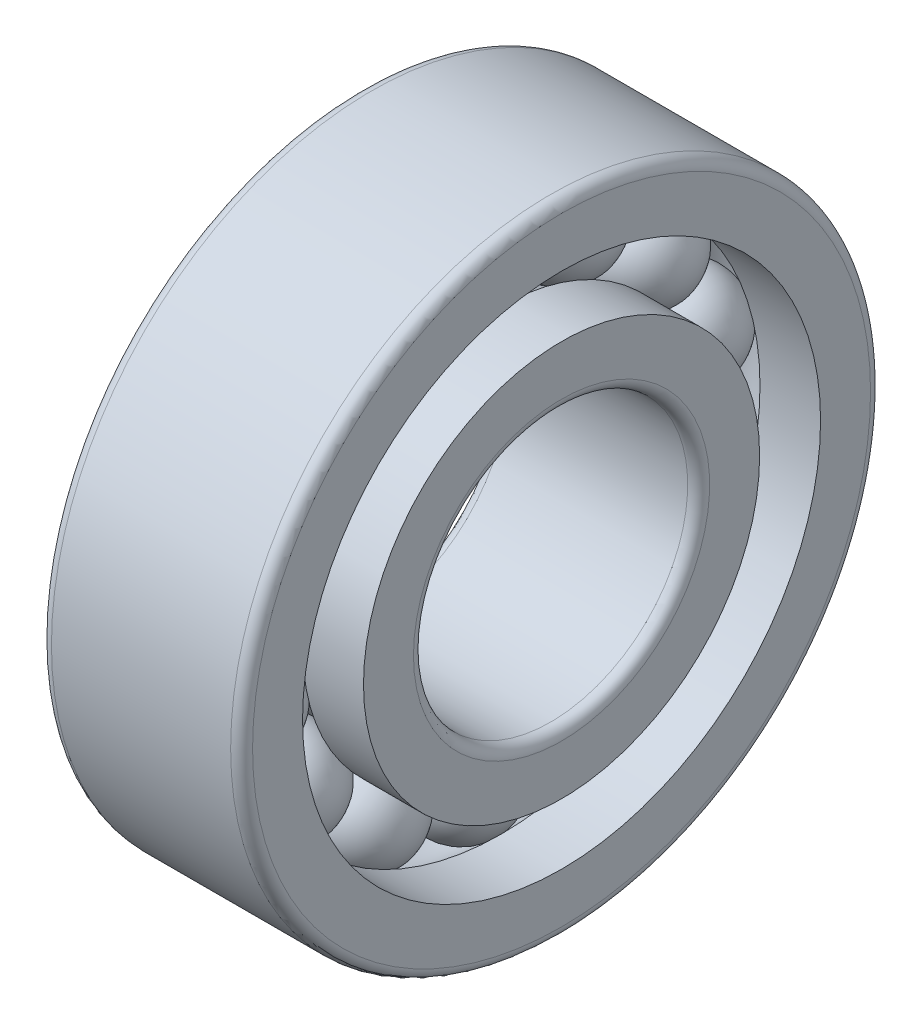
from build123d import *

# Parameters (mm, degrees)
PATTERN_CIRCULAR_5_COUNT = 14


with BuildPart() as part:
    # 草图2 → 旋转1 (revolve)
    with BuildSketch(Plane.XY, mode=Mode.PRIVATE) as revolve_1_sk:
        with BuildLine():
            Line((-5.2, 10.833333333), (-5.5, 10.833333333))
            Line((-5.5, 10.833333333), (-5.5, 10.233333333))
            Line((-5.5, 10.233333333), (-5.5, 8.1))
            ThreePointArc((-5.5, 8.1), (-5.324264069, 7.675735931), (-4.9, 7.5))
            Line((-4.9, 7.5), (4.9, 7.5))
            ThreePointArc((4.9, 7.5), (5.324264069, 7.675735931), (5.5, 8.1))
            Line((5.5, 8.1), (5.5, 10.233333333))
            Line((5.5, 10.233333333), (5.5, 10.833333333))
            Line((5.5, 10.833333333), (4.9, 10.833333333))
            Line((4.9, 10.833333333), (2.187400791, 10.833333333))
            ThreePointArc((2.187400791, 10.833333333), (0, 9.75), (-2.187400791, 10.833333333))
            Line((-2.187400791, 10.833333333), (-4, 10.833333333))
            Line((-4, 10.833333333), (-4, 10.233333333))
            Line((-4, 10.233333333), (-4.6, 10.233333333))
            Line((-4.6, 10.233333333), (-5.2, 10.833333333))
        make_face()
        with BuildLine():
            Line((-5.5, 14.166666667), (-5.2, 14.166666667))
            Line((-5.2, 14.166666667), (-4.6, 14.766666667))
            Line((-4.6, 14.766666667), (-4, 14.766666667))
            Line((-4, 14.766666667), (-4, 14.166666667))
            Line((-4, 14.166666667), (-2.187400791, 14.166666667))
            ThreePointArc((-2.187400791, 14.166666667), (0, 15.25), (2.187400791, 14.166666667))
            Line((2.187400791, 14.166666667), (5.5, 14.166666667))
            Line((5.5, 14.166666667), (5.5, 16.9))
            ThreePointArc((5.5, 16.9), (5.324264069, 17.324264069), (4.9, 17.5))
            Line((4.9, 17.5), (-4.9, 17.5))
            ThreePointArc((-4.9, 17.5), (-5.324264069, 17.324264069), (-5.5, 16.9))
            Line((-5.5, 16.9), (-5.5, 14.166666667))
        make_face()
    revolve(revolve_1_sk.sketch.rotate(Axis((-3.5, 0, 0), (1, 0, 0)), 90), axis=Axis((-3.5, 0, 0), (1, 0, 0)))


with BuildPart() as body_2:
    # 草图3 → 旋转2 (revolve)
    with BuildSketch(Plane.XY):
        with BuildLine():
            Line((-2.75, 12.5), (2.75, 12.5))
            ThreePointArc((2.75, 12.5), (0, 15.25), (-2.75, 12.5))
        make_face()
    revolve(axis=Axis((2.75, 12.5, 0), (1, 0, 0)))


with BuildPart() as body_3:
    # 草图4 → 旋转3 (revolve)
    with BuildSketch(Plane.XY, mode=Mode.PRIVATE) as revolve_3_sk:
        Polygon((-5.2, 14.166666667), (-5.2, 10.833333333), (-4.6, 10.233333333), (-4, 10.233333333), (-4, 10.833333333), (-4.6, 11.433333333), (-4.6, 13.566666667), (-4, 14.166666667), (-4, 14.766666667), (-4.6, 14.766666667), align=None)
    revolve(revolve_3_sk.sketch.rotate(Axis((-19.927092192, 0, 0), (1, 0, 0)), 90), axis=Axis((-19.927092192, 0, 0), (1, 0, 0)))


with BuildPart() as pattern_circular_5_1:
    # 阵列(圆周)5: pattern copy
    add(body_2.part.rotate(Axis((0, 0, 0), (1, 0, 0)), 1 * 360 / PATTERN_CIRCULAR_5_COUNT))


with BuildPart() as pattern_circular_5_2:
    # 阵列(圆周)5: pattern copy
    add(body_2.part.rotate(Axis((0, 0, 0), (1, 0, 0)), 2 * 360 / PATTERN_CIRCULAR_5_COUNT))


with BuildPart() as pattern_circular_5_3:
    # 阵列(圆周)5: pattern copy
    add(body_2.part.rotate(Axis((0, 0, 0), (1, 0, 0)), 3 * 360 / PATTERN_CIRCULAR_5_COUNT))


with BuildPart() as pattern_circular_5_4:
    # 阵列(圆周)5: pattern copy
    add(body_2.part.rotate(Axis((0, 0, 0), (1, 0, 0)), 4 * 360 / PATTERN_CIRCULAR_5_COUNT))


with BuildPart() as pattern_circular_5_5:
    # 阵列(圆周)5: pattern copy
    add(body_2.part.rotate(Axis((0, 0, 0), (1, 0, 0)), 5 * 360 / PATTERN_CIRCULAR_5_COUNT))


with BuildPart() as pattern_circular_5_6:
    # 阵列(圆周)5: pattern copy
    add(body_2.part.rotate(Axis((0, 0, 0), (1, 0, 0)), 6 * 360 / PATTERN_CIRCULAR_5_COUNT))


with BuildPart() as pattern_circular_5_7:
    # 阵列(圆周)5: pattern copy
    add(body_2.part.rotate(Axis((0, 0, 0), (1, 0, 0)), 7 * 360 / PATTERN_CIRCULAR_5_COUNT))


with BuildPart() as pattern_circular_5_8:
    # 阵列(圆周)5: pattern copy
    add(body_2.part.rotate(Axis((0, 0, 0), (1, 0, 0)), 8 * 360 / PATTERN_CIRCULAR_5_COUNT))


with BuildPart() as pattern_circular_5_9:
    # 阵列(圆周)5: pattern copy
    add(body_2.part.rotate(Axis((0, 0, 0), (1, 0, 0)), 9 * 360 / PATTERN_CIRCULAR_5_COUNT))


with BuildPart() as pattern_circular_5_10:
    # 阵列(圆周)5: pattern copy
    add(body_2.part.rotate(Axis((0, 0, 0), (1, 0, 0)), 10 * 360 / PATTERN_CIRCULAR_5_COUNT))


with BuildPart() as pattern_circular_5_11:
    # 阵列(圆周)5: pattern copy
    add(body_2.part.rotate(Axis((0, 0, 0), (1, 0, 0)), 11 * 360 / PATTERN_CIRCULAR_5_COUNT))


with BuildPart() as pattern_circular_5_12:
    # 阵列(圆周)5: pattern copy
    add(body_2.part.rotate(Axis((0, 0, 0), (1, 0, 0)), 12 * 360 / PATTERN_CIRCULAR_5_COUNT))


with BuildPart() as pattern_circular_5_13:
    # 阵列(圆周)5: pattern copy
    add(body_2.part.rotate(Axis((0, 0, 0), (1, 0, 0)), 13 * 360 / PATTERN_CIRCULAR_5_COUNT))


solid = Compound([part.part, body_2.part, body_3.part, pattern_circular_5_1.part, pattern_circular_5_2.part, pattern_circular_5_3.part, pattern_circular_5_4.part, pattern_circular_5_5.part, pattern_circular_5_6.part, pattern_circular_5_7.part, pattern_circular_5_8.part, pattern_circular_5_9.part, pattern_circular_5_10.part, pattern_circular_5_11.part, pattern_circular_5_12.part, pattern_circular_5_13.part])
